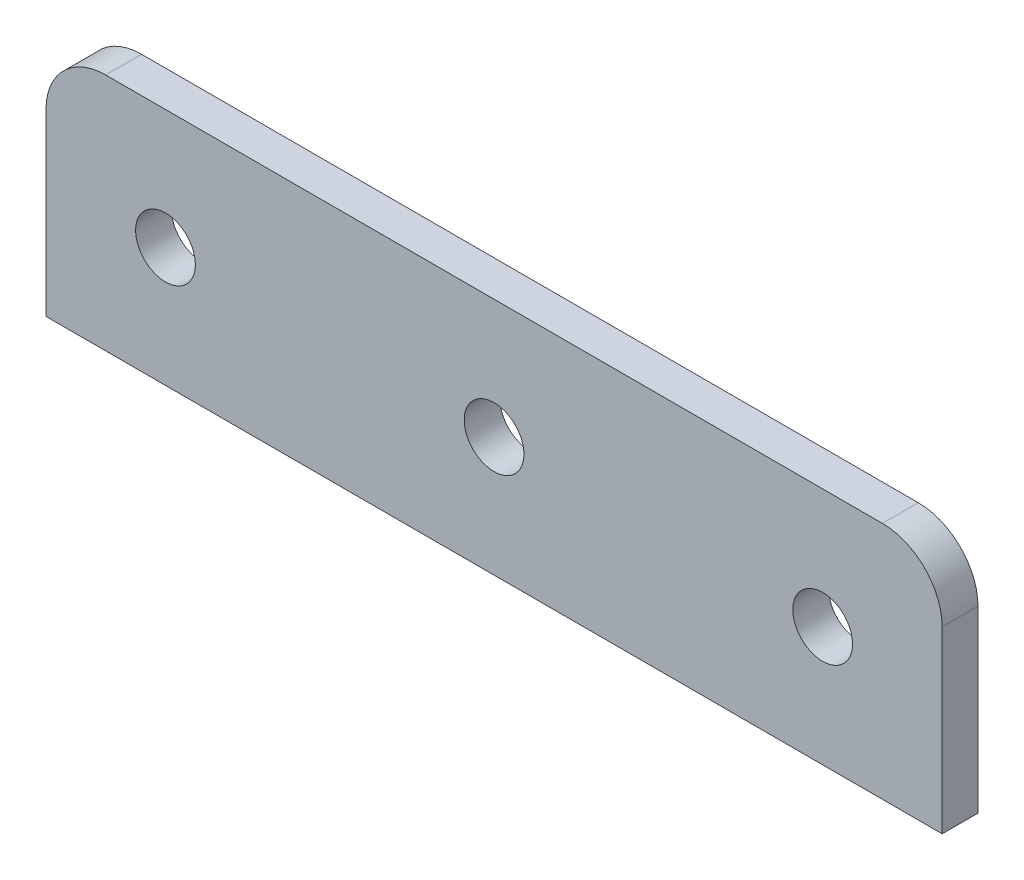
from build123d import *

# Parameters (mm, degrees)
SKETCH1_W           = 75
SKETCH1_H           = 20
SKETCH1_R           = 2.5
BOSS_EXTRUDE1_DEPTH = 3
FILLET1_R           = 5


with BuildPart() as part:
    # Sketch1 → Boss-Extrude1 (new body)
    with BuildSketch(Plane.XY):
        with Locations((37.5, -10)):
            Rectangle(SKETCH1_W, SKETCH1_H)
        with Locations((10, -10)):
            Circle(SKETCH1_R, mode=Mode.SUBTRACT)
        with Locations((65, -10)):
            Circle(SKETCH1_R, mode=Mode.SUBTRACT)
        with Locations((37.5, -10)):
            Circle(SKETCH1_R, mode=Mode.SUBTRACT)
    extrude(amount=BOSS_EXTRUDE1_DEPTH)

    # Fillet1
    fillet1_edges = [part.edges().sort_by_distance(p)[0] for p in [
        (0, 0, 1.5),
        (75, 0, 1.5),
    ]]
    fillet(fillet1_edges, radius=FILLET1_R)


solid = part.part
